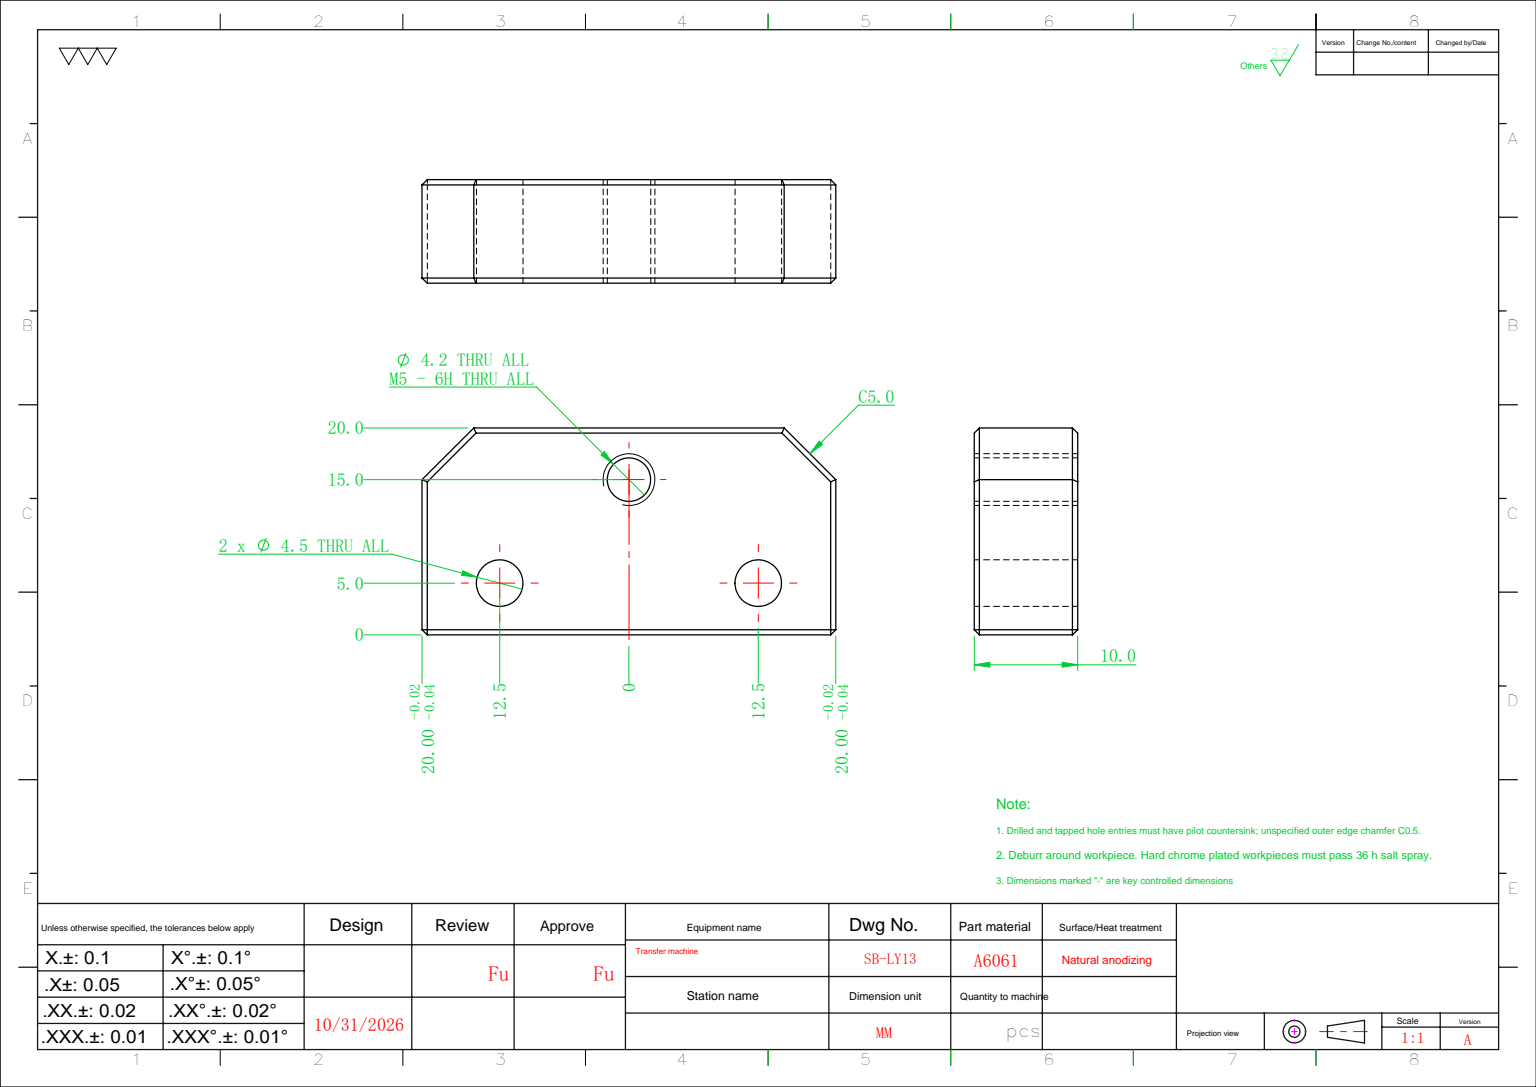
SolidWorks part; units mm, degrees
ref_plane "前视基准面" through (0, 0, 0) normal (0, 0, 1) x (1, 0, 0)
ref_plane "上视基准面" through (0, 0, 0) normal (0, 1, 0) x (1, 0, 0)
ref_plane "右视基准面" through (0, 0, 0) normal (1, 0, 0) x (0, 0, -1)
sketch "草图1" plane through (0, 0, 0) normal (0, 0, 1) x (1, 0, 0)
  line L1 (-20, -10) -> (20, -10)
  line L2 (-20, -10) -> (-20, 10)
  line L3 (-20, 10) -> (20, 10)
  line L4 (20, -10) -> (20, 10)
  line L5 (-20, -10) -> (20, 10) construction
  line L6 (-20, 10) -> (20, -10) construction
  point P0 (0, 0)
  dimension "D1" = 40
  dimension "D2" = 20
extrude "凸台-拉伸1" add sketch "草图1" along normal blind 10
hole_wizard "Ø4.5 (4.5) 直径孔1" positions "草图2" profile "草图3" hole size "Ø4.5" standard "ISO" end condition through all
sketch "草图2" plane through (0, 0, 10) normal (0, 0, 1) x (1, 0, 0)
  line L1 (0, 0) -> (0, 13.2503) construction
  line L3 (20, 10) -> (-20, 10) construction
  point P0 (12.5, 5)
  point P2 (-12.5, 5)
  dimension "D1" = 25
  dimension "D2" = 5
sketch "草图3" plane through (12.5, 5, 10) normal (1, 0, 0) x (0, -1, 0)
  line L0 (0, 0) -> (0, 10)
  line L1 (0, 10) -> (2.25, 10)
  line L2 (2.25, 10) -> (2.25, 0)
  line L5 (2.25, 0) -> (0, 0)
  line L11 (0, -6.35) -> (0, 107.95) construction
  dimension "通孔孔直径" = 4.5
  dimension "通孔孔深度" = 10
hole_wizard "M5 螺纹孔1" positions "草图4" profile "草图5" tap size "M5" standard "ISO" end condition through all
sketch "草图4" plane through (0, 0, 10) normal (0, 0, 1) x (1, 0, 0)
  line L0 (0, 0) -> (0, -12.9022) construction
  circle A0 centre (-12.5, 5) radius 2.25 construction
  point P0 (0, -5)
  dimension "D1" = 10
sketch "草图5" plane through (0, -5, 10) normal (1, 0, 0) x (0, -1, 0)
  line L0 (0, 0) -> (0, 10)
  line L1 (0, 10) -> (2.1, 10)
  line L2 (2.1, 10) -> (2.1, 0)
  line L5 (2.1, 0) -> (0, 0)
  line L11 (0, -6.35) -> (0, 107.95) construction
  dimension "通孔螺纹孔钻头直径" = 4.2
  dimension "通孔螺纹孔钻头深度" = 10
cosmetic thread "孔螺蚊线1" parameters "D2"=5
chamfer "倒角1" distance 5 angle 45 2 edges at (-20, -10, 5) (20, -10, 5)
chamfer "倒角2" distance 0.5 angle 45 14 edges at (20, 10, 5) (17.5, -7.5, 0) (20, 2.5, 0) (0, 10, 0) (0, -10, 0) (-17.5, -7.5, 0) (-20, 2.5, 0) (-20, 10, 5) (0, 10, 10) (20, 2.5, 10) (17.5, -7.5, 10) (0, -10, 10) (-17.5, -7.5, 10) (-20, 2.5, 10)
